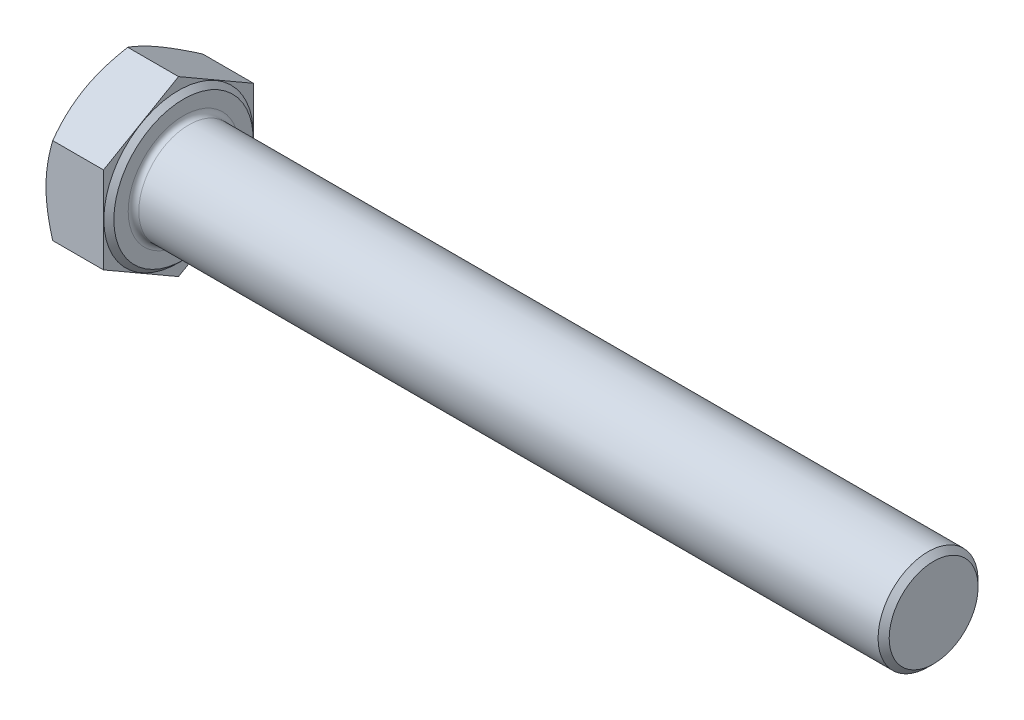
SolidWorks part; units mm, degrees
material "Q235"
ref_plane "Front Plane" through (0, 0, 0) normal (0, 0, 1) x (1, 0, 0)
ref_plane "Top Plane" through (0, 0, 0) normal (0, 1, 0) x (1, 0, 0)
ref_plane "Right Plane" through (0, 0, 0) normal (1, 0, 0) x (0, 0, -1)
sketch "Sketch1" plane through (0, 0, 0) normal (0, 0, 1) x (1, 0, 0)
  line L0 (0, 0) -> (130, 0) construction
  line L1 (0, 0) -> (0, 13.375)
  line L2 (0, 13.375) -> (10, 13.375)
  line L3 (10, 13.375) -> (10, 0)
  line L4 (10, 8) -> (130, 8)
  line L5 (130, 8) -> (130, 0)
  line L6 (0, 12) -> (0.7939, 13.375)
  line L7 (126, 8) -> (126, 0)
  line L8 (16, 8) -> (16, 0)
  line L9 (10, 7.3505) -> (130, 7.3505)
  line L10 (130, 6.9175) -> (10, 6.9175)
  line L11 (9.2, 11.945) -> (10, 11.145)
  line L12 (9.2, 13.375) -> (9.2, 0)
  line L13 (9.9, 11.245) -> (9.9, 0) construction
  arc A0 (10, 8.85) -> (10.85, 8) centre (10.85, 8.85) ccw
  point P12 (128, 0)
  point P13 (3.13, 13.375)
  point P14 (10, 8.85)
  point P24 (10, 11.245)
  dimension "D1" = 0.1
  dimension "r" = 0.85
  dimension "k" = 10
  dimension "D2" = 45
  dimension "β" = 30
  dimension "e" = 26.75
  dimension "s" = 24
  dimension "d" = 16
  dimension "l" = 120
  dimension "D52" = 4
  dimension "P" = 2
  dimension "kw" = 6.87
  dimension "da" = 17.7
  dimension "a" = 6
  dimension "ds" = 14.701
  dimension "D61" = 13.835
  dimension "dw" = 22.49
  dimension "c" = 0.8
sketch "Sketch2" plane through (0, 0, 0) normal (1, 0, 0) x (0, 0, -1)
  line L1 (0, 13.8564) -> (-12, 6.9282)
  line L2 (-12, 6.9282) -> (-12, -6.9282)
  line L3 (-12, -6.9282) -> (0, -13.8564)
  line L4 (0, -13.8564) -> (12, -6.9282)
  line L5 (12, -6.9282) -> (12, 6.9282)
  line L6 (12, 6.9282) -> (0, 13.8564)
  circle A0 centre (0, 0) radius 12 construction
sketch "Sketch3" plane through (0, 0, 0) normal (1, 0, 0) x (0, 0, -1)
  line L0 (12, 6.9282) -> (0, 13.8564) construction
  line L1 (0, 13.8564) -> (-12, 6.9282) construction
  line L2 (-12, 6.9282) -> (-12, -6.9282) construction
  line L3 (12, -6.9282) -> (12, 6.9282) construction
  line L4 (0, -13.8564) -> (12, -6.9282) construction
  line L5 (-12, -6.9282) -> (0, -13.8564) construction
  line L6 (12, 6.9282) -> (0, 13.8564)
  line L7 (0, 13.8564) -> (-12, 6.9282)
  line L8 (-12, 6.9282) -> (-12, -6.9282)
  line L9 (12, -6.9282) -> (12, 6.9282)
  line L10 (0, -13.8564) -> (12, -6.9282)
  line L11 (-12, -6.9282) -> (0, -13.8564)
extrude "Boss-Extrude1" add sketch "Sketch3" along normal up to vertex (10 mm away) up to point (10, 13.375, 0)
sketch "Sketch4" plane through (0, 0, 0) normal (-1, 0, 0) x (0, 0, 1)
  circle A0 centre (0, 0) radius 12 construction
  circle A1 centre (0, 0) radius 12
  circle A2 centre (0, 0) radius 26.75
  dimension "D1" = 53.5
extrude "Cut-Extrude1" cut sketch "Sketch4" against normal blind 1.25 draft 60
sketch "Sketch5" plane through (0, 0, 0) normal (0, 0, 1) x (1, 0, 0)
  line L0 (10, 8) -> (130, 8) construction
  line L1 (130, 8) -> (130, 0) construction
  line L2 (0, 0) -> (130, 0) construction
  line L3 (10.85, 8) -> (130, 8)
  line L4 (130, 8) -> (130, 0)
  line L5 (10, 0) -> (130, 0)
  line L6 (10, 8.85) -> (10, 0)
  arc A0 (10, 8.85) -> (10.85, 8) centre (10.85, 8.85) ccw construction
  arc A1 (10, 8.85) -> (10.85, 8) centre (10.85, 8.85) ccw
revolve "Revolve1" add sketch "Sketch5" angle 360 about L5
cosmetic thread "Cosmetic Thread2" parameters "D1"=64, "D2"=13.835
chamfer "Chamfer2" distance 0.8889 angle 45 1 edges at (130, 0, 8)
sketch "Sketch7" plane through (0, 0, 0) normal (0, 0, 1) x (1, 0, 0)
  line L0 (10, 11.145) -> (9.2, 11.945)
  line L1 (9.2, 11.945) -> (9.2, 26.75)
  line L2 (9.2, 26.75) -> (10, 26.75)
  line L3 (10, 26.75) -> (10, 11.145)
  line L4 (0, 0) -> (130, 0) construction
  line L5 (0, 0) -> (130, 0) construction
  dimension "D1" = 53.5
revolve "Cut-Revolve1" cut sketch "Sketch7" angle 360 mid plane about L5
sketch "Sketch6" [suppressed] plane through (0, 0, 0) normal (0, 0, 1) x (1, 0, 0)
  line L0 (9.3, 0) -> (9.3, 4) construction
  line L1 (9.3, 4) -> (75.3, 4)
  line L2 (75.3, 4) -> (75.3, 0)
  line L3 (9.3, 4) -> (5.9719, 3.5984)
  line L5 (5.3, 3.5941) -> (75.3, 3.5941) construction
  line L6 (5.3, 7.19) -> (5.3, 0) construction
  line L7 (5.3, 4.1941) -> (5.3, 0)
  line L8 (5.3, 0) -> (75.3, 0)
  arc A0 (5.9719, 3.5984) -> (5.3, 4.1941) centre (5.9, 4.1941) cw
  arc A1 (5.3, 4.6) -> (5.9, 4) centre (5.9, 4.6) ccw construction
revolve "Revolve2" add sketch "Sketch6" angle 360 about L8
cosmetic thread "Cosmetic Thread1" [suppressed] parameters "D1"=44, "D2"=13.835
chamfer "Chamfer1" [suppressed] distance 0.8889 angle 45
sketch "Sketch8" [suppressed] plane through (0, 0, 0) normal (0, 0, 1) x (1, 0, 0)
  line L0 (5.3, 5.715) -> (4.7, 6.315)
  line L1 (4.7, 6.315) -> (4.7, 14.38)
  line L2 (4.7, 14.38) -> (5.3, 14.38)
  line L3 (5.3, 14.38) -> (5.3, 5.715)
  line L4 (0, 0) -> (75.3, 0) construction
  line L5 (0, 0) -> (75.3, 0) construction
  dimension "D1" = 53.5
revolve "Cut-Revolve2" [suppressed] cut sketch "Sketch8" angle 360 mid plane about L5
